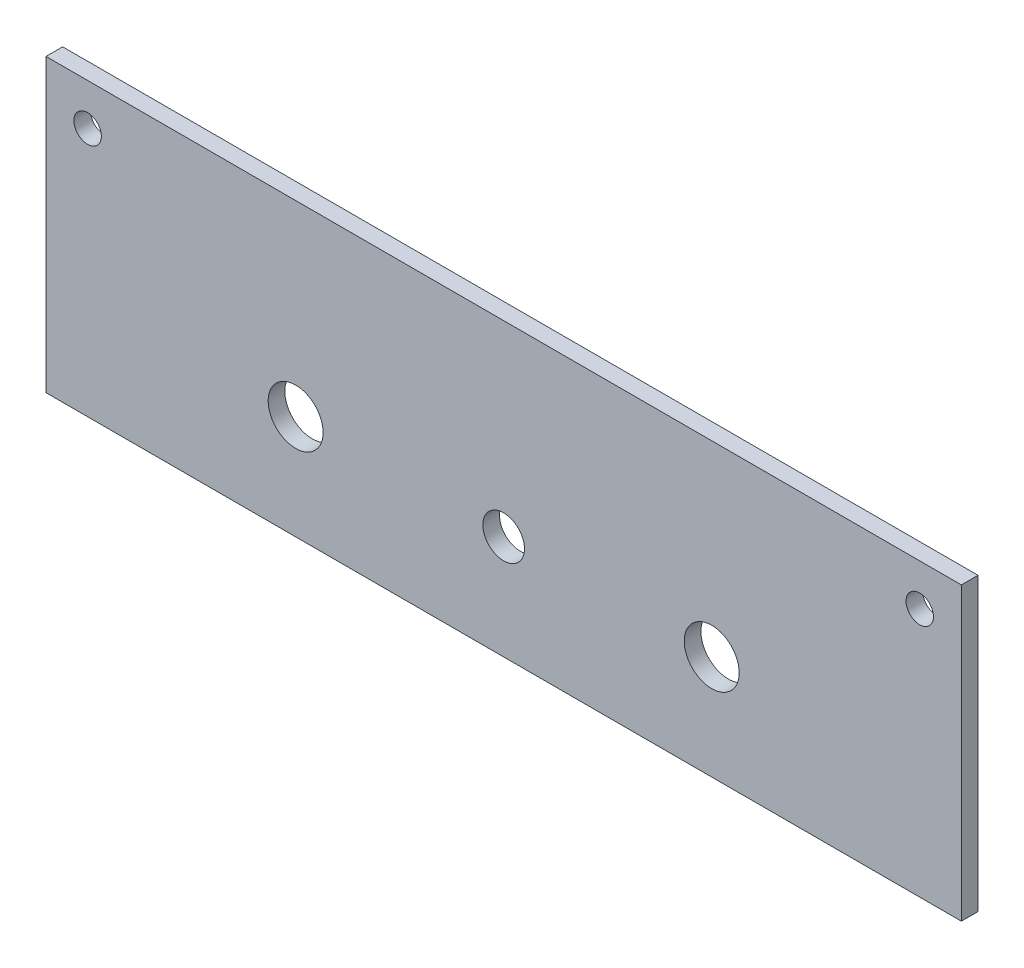
SolidWorks part; units mm, degrees
ref_plane "前视基准面" through (0, 0, 0) normal (0, 0, 1) x (1, 0, 0)
ref_plane "上视基准面" through (0, 0, 0) normal (0, 1, 0) x (1, 0, 0)
ref_plane "右视基准面" through (0, 0, 0) normal (1, 0, 0) x (0, 0, -1)
sketch "草图1" plane through (0, 0, 0) normal (0, 0, 1) x (1, 0, 0)
  line L0 (-25, 0) -> (25, 0) construction
  line L1 (55, -12.5) -> (-55, -12.5)
  line L2 (55, -12.5) -> (55, 12.5)
  line L3 (55, 12.5) -> (-55, 12.5)
  line L4 (-55, -12.5) -> (-55, 12.5)
  line L5 (55, -12.5) -> (-55, 12.5) construction
  line L6 (55, 12.5) -> (-55, -12.5) construction
  circle A0 centre (-25, 0) radius 3.3
  circle A1 centre (25, 0) radius 3.3
  point P0 (0, 0)
  dimension "D1" = 50
  dimension "D2" = 6.6
  dimension "D3" = 25
  dimension "D4" = 110
extrude "凸台-拉伸1" add sketch "草图1" along normal mid plane 2
sketch "草图2" plane through (0, 0, 1) normal (0, 0, 1) x (1, 0, 0)
  circle A0 centre (0, 0) radius 2.5
  dimension "D1" = 5
extrude "切除-拉伸1" cut sketch "草图2" against normal blind 10
sketch "草图3" plane through (0, 12.5, 0) normal (0, 1, 0) x (1, 0, 0)
  line L4 (55, 1) -> (-55, 1)
  line L5 (-55, 1) -> (-55, -1)
  line L6 (-55, -1) -> (55, -1)
  line L7 (55, -1) -> (55, 1)
  line L8 (55, 1) -> (-55, 1)
  line L9 (-55, 1) -> (-55, -1)
  line L10 (-55, -1) -> (55, -1)
  line L11 (55, -1) -> (55, 1)
  dimension "D1" = 0
extrude "凸台-拉伸2" add sketch "草图3" along normal blind 10
sketch "草图4" plane through (0, 0, -1) normal (0, 0, -1) x (-1, 0, 0)
  line L0 (-55, 17.5) -> (-50, 17.5) construction
  line L1 (-55, -12.5) -> (-55, 22.5) construction
  line L2 (-50, 17.5) -> (50, 17.5) construction
  line L3 (50, 17.5) -> (55, 17.5) construction
  line L4 (55, 22.5) -> (55, -12.5) construction
  line L5 (-55, 22.5) -> (55, 22.5) construction
  circle A0 centre (-50, 17.5) radius 1.65
  circle A1 centre (50, 17.5) radius 1.65
  dimension "D3" = 3.3
  dimension "D1" = 5
  dimension "D2" = 5
extrude "切除-拉伸2" cut sketch "草图4" against normal blind 10
